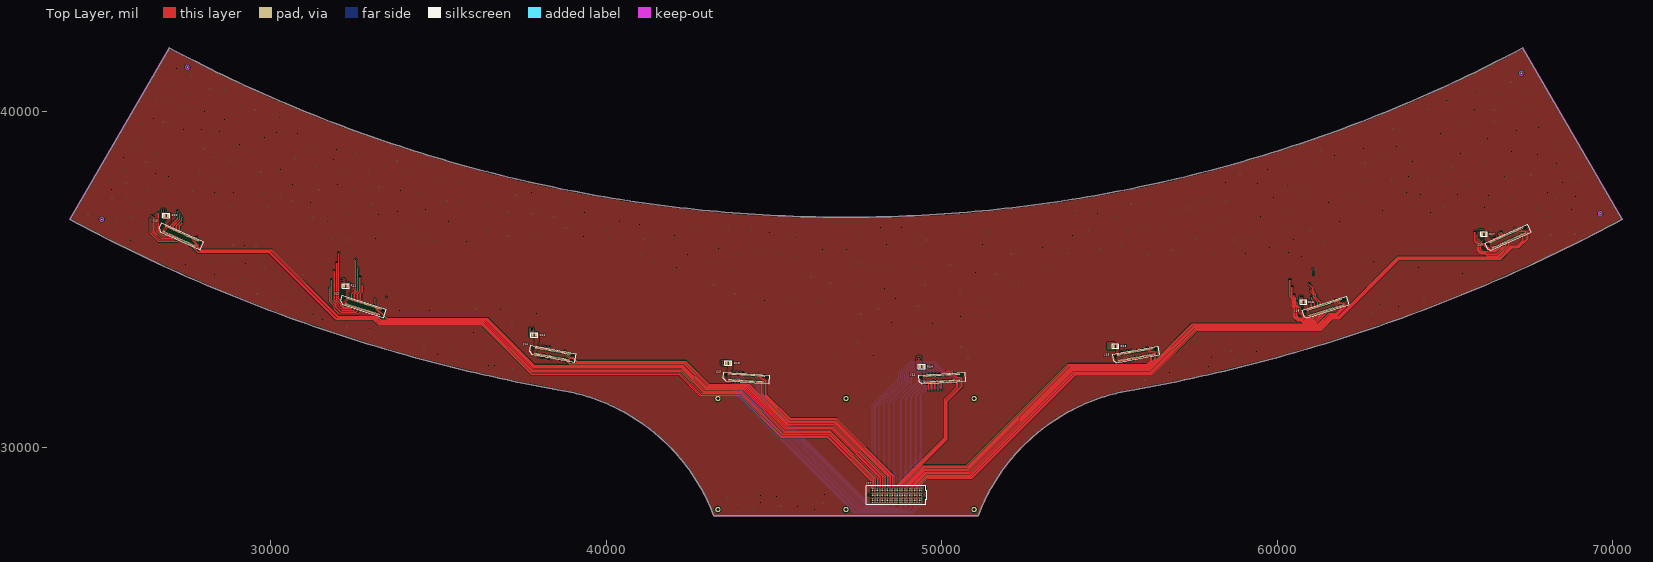
[diagram p0: Top Layer view]
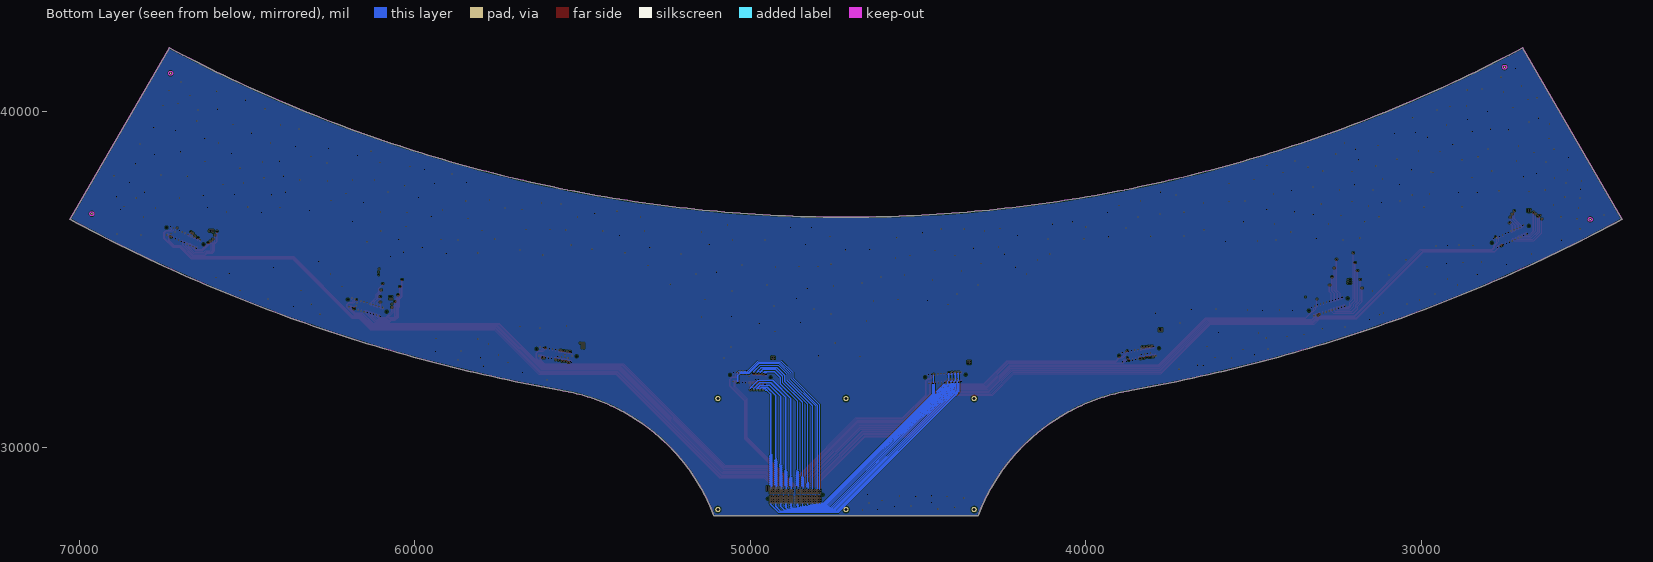
[diagram p1: Bottom Layer view, seen from below]
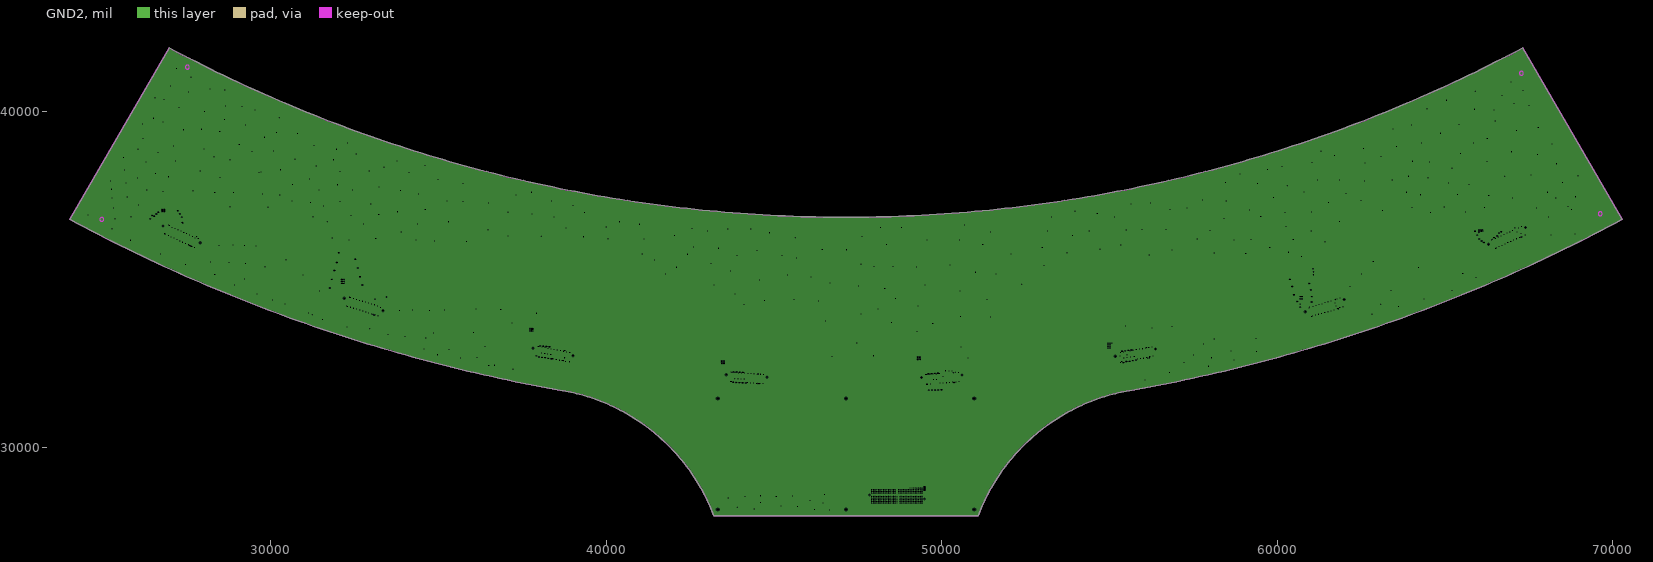
[diagram p2: GND2, clearances drawn from the general rule]
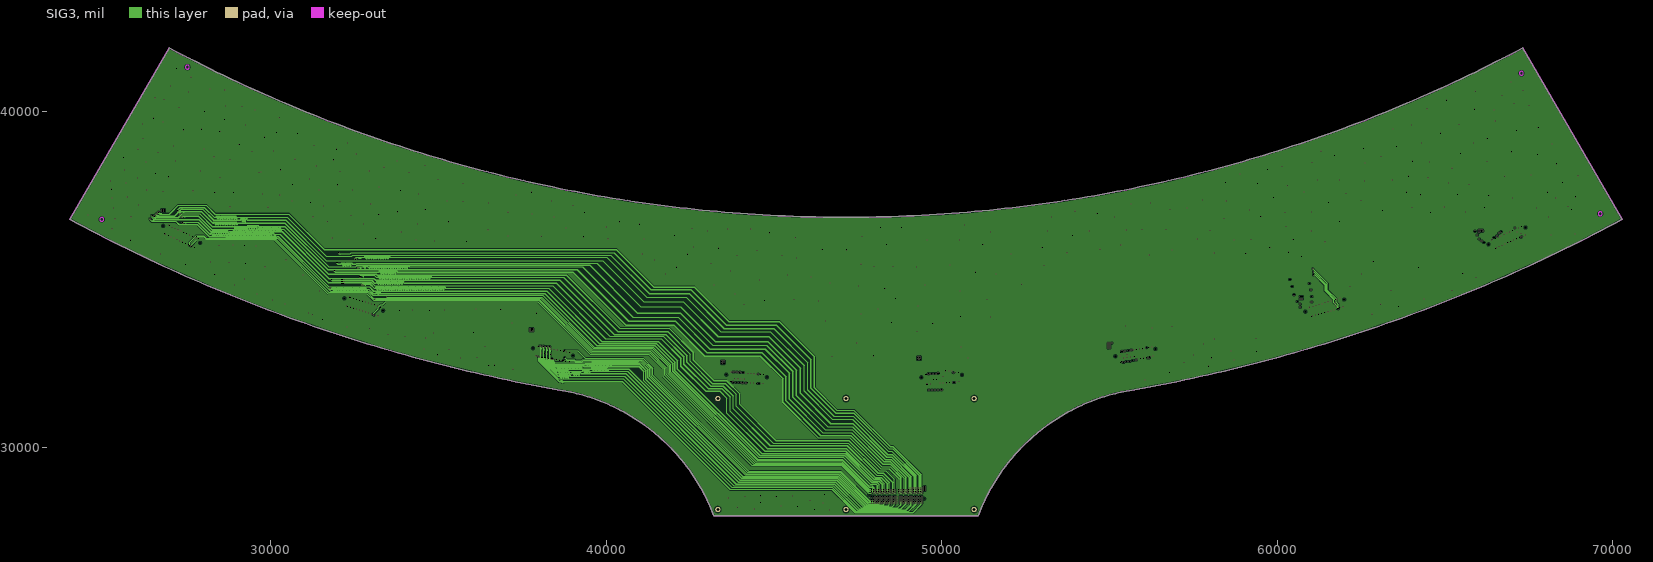
[diagram p3: SIG3]
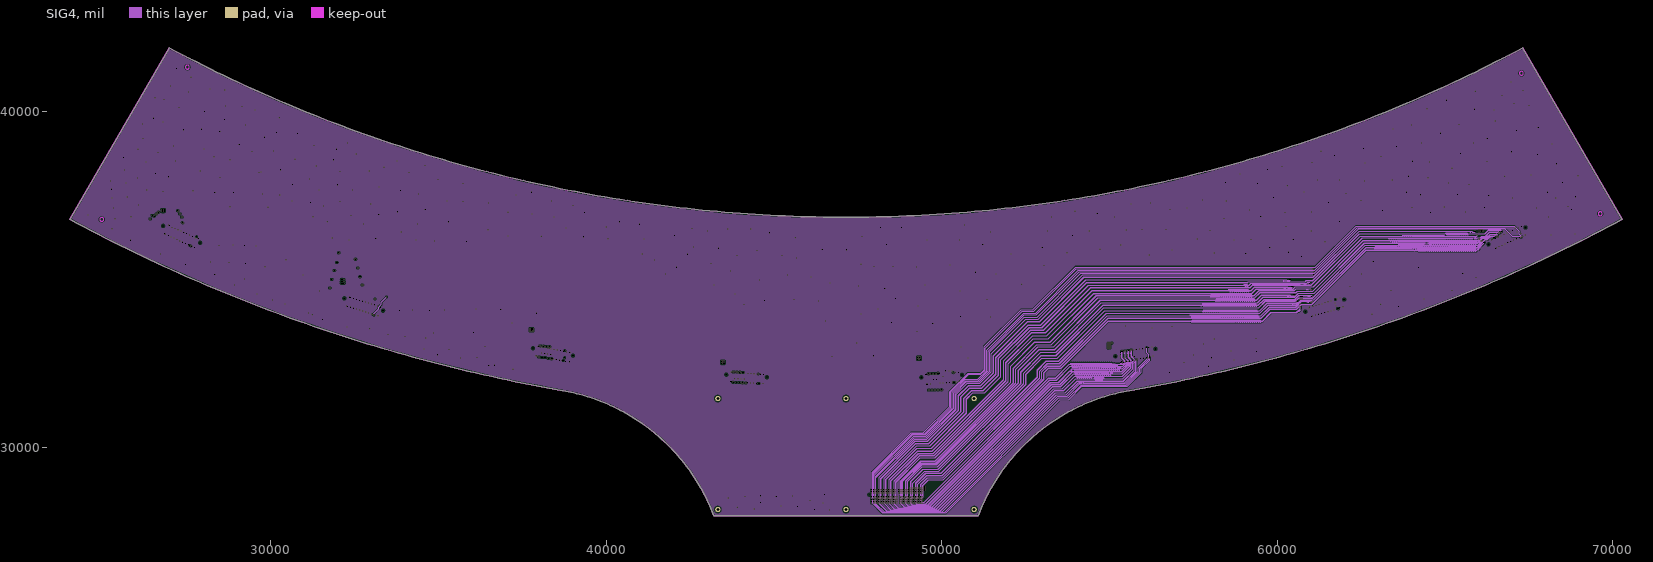
[diagram p4: SIG4]
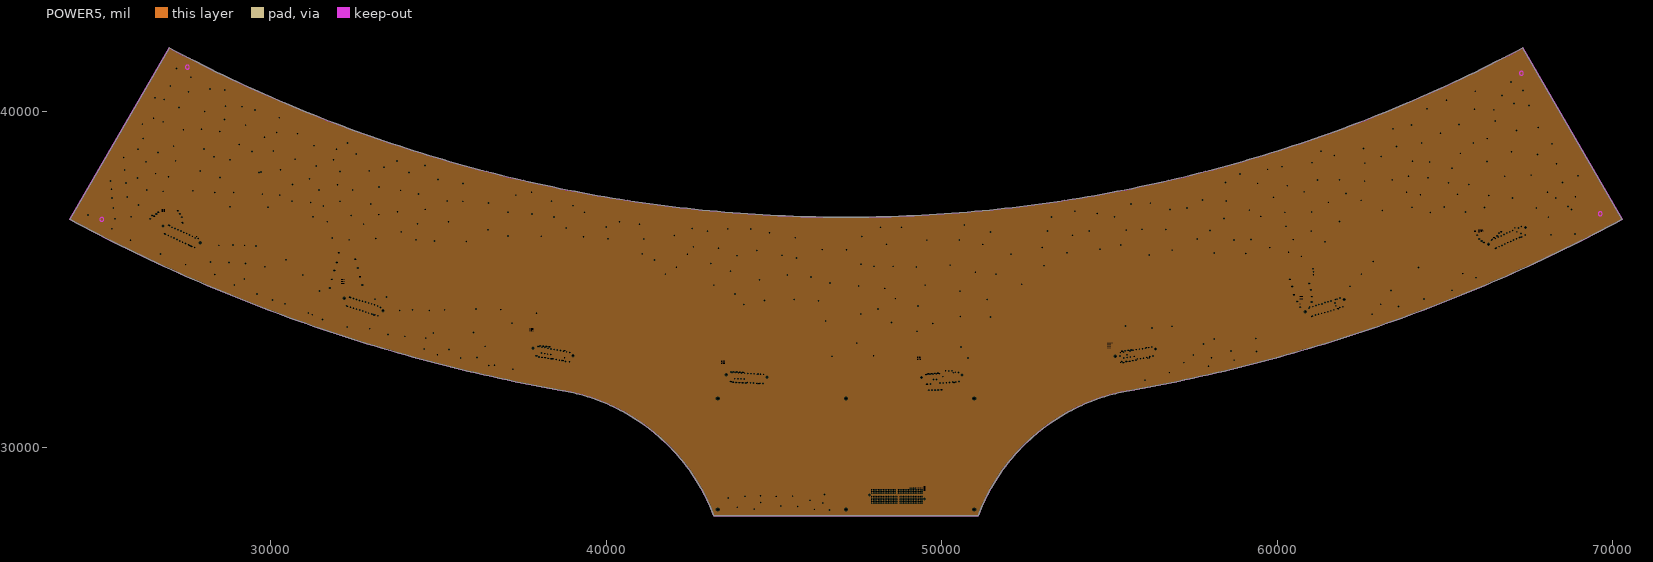
[diagram p5: POWER5, clearances drawn from the general rule]
# Altium PCB MISC86329.PcbDoc (part 1 of 11)
Units mil, origin at the board's own origin, x right, y up, seen from the top; angles counter-clockwise.
Board outline 46247.15 x 13937.21 mil, 6 copper layers (Top Layer, GND2, SIG3, SIG4, POWER5, Bottom Layer); 17 components, 210 nets, 908 pads, 1109 vias.

## Layer stack, top to bottom (the 12.6 mil dielectric is the usual default, probably not edited)
Top Layer: signal copper 1.4
Dielectric: core 12.6, FR-4, Dk 4.8
GND2: plane copper 1.4, net DGND
Dielectric: prepreg 12.6, FR-4, Dk 4.8
SIG3: signal copper 1.4
Dielectric: core 12.6, FR-4, Dk 4.8
SIG4: signal copper 1.4
Dielectric: prepreg 12.6, FR-4, Dk 4.8
POWER5: plane copper 1.4, net 5V_OUT
Dielectric: core 12.6, FR-4, Dk 4.8
Bottom Layer: signal copper 1.4

## Board outline
24025.43,36800.52 ccw(c47149,79657.81) 38712.02,31696.74 38711.64,31696.8 cw(c37688.49,25880.6) 43212,27970.07 43211.99,27970.1 51086.01,27970.1 51086,27970.07 cw(c56609.51,25880.6) 55586.37,31696.8 55585.98,31696.74 ccw(c47149,79657.81) 70272.58,36800.52 70272.27,36800.35 67306.49,41907.14 67306.76,41907.28 cw(c47149,79657.81) 26991.25,41907.28 26991.51,41907.14

## Design rules (kind name [scope] priority, off if disabled: settings)
Clearance [All] p1: gap=5
DiffPairsRouting [All] p1: maxlimit=5 minlimit=5 mostfreqgap=5 maxuncoupledlength=500
HoleToHoleClearance [All] p1: gap=0 allowstackedmicrovias=TRUE
MinimumSolderMaskSliver [All] p1: minsoldermaskwidth=0
PlaneClearance [All] p1: clearance=20
PlaneConnect [All] p1: planeconnectstyle=Direct reliefexpansion=20 reliefentries=4 reliefconductorwidth=10 reliefairgap=10
PolygonConnect PolygonConnect_1 [isvia] p1: connectstyle=Direct reliefconductorwidth=10 reliefentries=4 polygonreliefangle="90 Angle"
PolygonConnect [All] p2: connectstyle=Relief reliefconductorwidth=10 reliefentries=4 polygonreliefangle="90 Angle"
RoutingVias [All] p1: holewidth=12 width=24 viastyle="Through Hole" minholewidth=12 minwidth=24 maxholewidth=12 maxwidth=24
SilkToSilkClearance [All] p1: silktosilkclearance=0
SilkscreenOverComponentPads [All] p1: minsilkscreentomaskgap=0
SolderMaskExpansion [All] p1: expansion=4
Width [All] p1: maxlimit=20 minlimit=5 preferedwidth=5 minimp=50.000000 maximp=50.000000 favimp=50.000000
21 further rules are at their usual default settings.

## Classes and differential pairs
differential pair NewDifferentialPair1: +CLKM_CH0 -CLKP_CH0
differential pair NewDifferentialPair2: +CLKM_CH1 -CLKP_CH1
differential pair NewDifferentialPair3: +CLKM_CH2 -CLKP_CH2
differential pair NewDifferentialPair4: +CLKM_CH3 -CLKP_CH3
differential pair NewDifferentialPair5: +CLKM_CH4 -CLKP_CH4
differential pair NewDifferentialPair6: +CLKM_CH5 -CLKP_CH5
differential pair NewDifferentialPair7: +CLKM_CH6 -CLKP_CH6
differential pair NewDifferentialPair8: +CLKM_CH7 -CLKP_CH7
differential pair NewDifferentialPair9: +DATAIN0N_CH0 -DATAIN0P_CH0
differential pair NewDifferentialPair10: +DATAIN0N_CH1 -DATAIN0P_CH1
differential pair NewDifferentialPair11: +DATAIN0N_CH2 -DATAIN0P_CH2
differential pair NewDifferentialPair12: +DATAIN0N_CH3 -DATAIN0P_CH3
differential pair NewDifferentialPair13: +DATAIN0N_CH4 -DATAIN0P_CH4
differential pair NewDifferentialPair14: +DATAIN0N_CH5 -DATAIN0P_CH5
differential pair NewDifferentialPair15: +DATAIN0N_CH6 -DATAIN0P_CH6
differential pair NewDifferentialPair16: +DATAIN0N_CH7 -DATAIN0P_CH7
differential pair NewDifferentialPair17: +DATAIN1N_CH0 -DATAIN1P_CH0
differential pair NewDifferentialPair18: +DATAIN1N_CH1 -DATAIN1P_CH1
differential pair NewDifferentialPair19: +DATAIN1N_CH2 -DATAIN1P_CH2
differential pair NewDifferentialPair20: +DATAIN1N_CH3 -DATAIN1P_CH3
differential pair NewDifferentialPair21: +DATAIN1N_CH4 -DATAIN1P_CH4
differential pair NewDifferentialPair22: +DATAIN1N_CH5 -DATAIN1P_CH5
differential pair NewDifferentialPair23: +DATAIN1N_CH6 -DATAIN1P_CH6
differential pair NewDifferentialPair24: +DATAIN1N_CH7 -DATAIN1P_CH7
differential pair NewDifferentialPair25: +DATAIN2N_CH0 -DATAIN2P_CH0
differential pair NewDifferentialPair26: +DATAIN2N_CH1 -DATAIN2P_CH1
differential pair NewDifferentialPair27: +DATAIN2N_CH2 -DATAIN2P_CH2
differential pair NewDifferentialPair28: +DATAIN2N_CH3 -DATAIN2P_CH3
differential pair NewDifferentialPair29: +DATAIN2N_CH4 -DATAIN2P_CH4
differential pair NewDifferentialPair30: +DATAIN2N_CH5 -DATAIN2P_CH5
differential pair NewDifferentialPair31: +DATAIN2N_CH6 -DATAIN2P_CH6
differential pair NewDifferentialPair32: +DATAIN2N_CH7 -DATAIN2P_CH7
differential pair NewDifferentialPair33: +DATAIN3N_CH0 -DATAIN3P_CH0
differential pair NewDifferentialPair34: +DATAIN3N_CH1 -DATAIN3P_CH1
differential pair NewDifferentialPair35: +DATAIN3N_CH2 -DATAIN3P_CH2
differential pair NewDifferentialPair36: +DATAIN3N_CH3 -DATAIN3P_CH3
differential pair NewDifferentialPair37: +DATAIN3N_CH4 -DATAIN3P_CH4
differential pair NewDifferentialPair38: +DATAIN3N_CH5 -DATAIN3P_CH5
differential pair NewDifferentialPair39: +DATAIN3N_CH6 -DATAIN3P_CH6
differential pair NewDifferentialPair40: +DATAIN3N_CH7 -DATAIN3P_CH7
differential pair NewDifferentialPair41: +DATAIN4N_CH0 -DATAIN4P_CH0
differential pair NewDifferentialPair42: +DATAIN4N_CH1 -DATAIN4P_CH1
differential pair NewDifferentialPair43: +DATAIN4N_CH2 -DATAIN4P_CH2
differential pair NewDifferentialPair44: +DATAIN4N_CH3 -DATAIN4P_CH3
differential pair NewDifferentialPair45: +DATAIN4N_CH4 -DATAIN4P_CH4
differential pair NewDifferentialPair46: +DATAIN4N_CH5 -DATAIN4P_CH5
differential pair NewDifferentialPair47: +DATAIN4N_CH6 -DATAIN4P_CH6
differential pair NewDifferentialPair48: +DATAIN4N_CH7 -DATAIN4P_CH7
differential pair NewDifferentialPair49: +DATAIN5N_CH0 -DATAIN5P_CH0
differential pair NewDifferentialPair50: +DATAIN5N_CH1 -DATAIN5P_CH1
differential pair NewDifferentialPair51: +DATAIN5N_CH2 -DATAIN5P_CH2
differential pair NewDifferentialPair52: +DATAIN5N_CH3 -DATAIN5P_CH3
differential pair NewDifferentialPair53: +DATAIN5N_CH4 -DATAIN5P_CH4
differential pair NewDifferentialPair54: +DATAIN5N_CH5 -DATAIN5P_CH5
differential pair NewDifferentialPair55: +DATAIN5N_CH6 -DATAIN5P_CH6
differential pair NewDifferentialPair56: +DATAIN5N_CH7 -DATAIN5P_CH7
differential pair NewDifferentialPair57: +DATAIN6N_CH0 -DATAIN6P_CH0
differential pair NewDifferentialPair58: +DATAIN6N_CH1 -DATAIN6P_CH1
differential pair NewDifferentialPair59: +DATAIN6N_CH2 -DATAIN6P_CH2
differential pair NewDifferentialPair60: +DATAIN6N_CH3 -DATAIN6P_CH3
differential pair NewDifferentialPair61: +DATAIN6N_CH4 -DATAIN6P_CH4
differential pair NewDifferentialPair62: +DATAIN6N_CH5 -DATAIN6P_CH5
differential pair NewDifferentialPair63: +DATAIN6N_CH6 -DATAIN6P_CH6
differential pair NewDifferentialPair64: +DATAIN6N_CH7 -DATAIN6P_CH7
differential pair NewDifferentialPair65: +DATAIN7N_CH0 -DATAIN7P_CH0
differential pair NewDifferentialPair66: +DATAIN7N_CH1 -DATAIN7P_CH1
differential pair NewDifferentialPair67: +DATAIN7N_CH2 -DATAIN7P_CH2
differential pair NewDifferentialPair68: +DATAIN7N_CH3 -DATAIN7P_CH3
differential pair NewDifferentialPair69: +DATAIN7N_CH4 -DATAIN7P_CH4
differential pair NewDifferentialPair70: +DATAIN7N_CH5 -DATAIN7P_CH5
differential pair NewDifferentialPair71: +DATAIN7N_CH6 -DATAIN7P_CH6
differential pair NewDifferentialPair72: +DATAIN7N_CH7 -DATAIN7P_CH7

## Components (designator, comment, footprint, x,y, rotation, side; value= is the part's Value field where it differs from the comment)
J10 "ERF8-035-XX.X-X-DV" ERF8-035-XX.X-X-DV 27328.13,36298.88 r155.43 top
J11 "ERF8-035-XX.X-X-DV" ERF8-035-XX.X-X-DV 50003.99,32068.81 r183.43 top
J12 "ERF8-035-XX.X-X-DV" ERF8-035-XX.X-X-DV 32759.99,34206.52 r162.43 top
J13 "ERF8-035-XX.X-X-DV" ERF8-035-XX.X-X-DV 44183.07,32075.6 r176.43 top
J14 "ERF8-035-XX.X-X-DV" ERF8-035-XX.X-X-DV 38406.36,32791.72 r169.43 top locked
J15 "ERF8-035-XX.X-X-DV" ERF8-035-XX.X-X-DV 55782.35,32771.47 r190.43 top
J16 "ERF8-035-XX.X-X-DV" ERF8-035-XX.X-X-DV 61432.01,34173.09 r197.43 top
J17 "SEAF-30-XX.X-XX-10-X-A" SEAF-30-XX.X-XX-10-X-A 48662.89,28593.8 r0 top locked
J18 "ERM8-035-XX.X-X-DV" ERF8-035-XX.X-X-DV 66868.74,36252.79 r204.43 top
R10 "100R" R1210 26890,36920 r180 top
R11 "100R" R1210 32240,34820 r180 top
R12 "100R" R1210 37860,33360 r180 top
R13 "100R" R1210 43640,32520 r180 top
R14 "100R" R1210 49409,32421 r180 top
R15 "100R" R1210 55180,33020 r180 top
R16 "100R" R1210 60780,34340 r180 top
R17 "100R" R1210 66160,36360 r180 top

## Footprints (in the part's own frame and the unit in brackets; to place one, negate y for a bottom-side part, rotate by r counter-clockwise, add the part's x,y. Pads: shape width x height; smd on the part's side, far side on the other; paste and mask are expansions set on the pad)
ERF8-035-XX.X-X-DV [mm]
  rect 0.5x1.1 smd mask+0.05: 1(13.6,2.25) 2(13.6,-2.25) 3(12.8,2.25) 4(12.8,-2.25) 5(12,2.25) 6(12,-2.25) 7(11.2,2.25) 8(11.2,-2.25) 9(10.4,2.25) 10(10.4,-2.25) 11(9.6,2.25) 12(9.6,-2.25) 13(8.8,2.25) 14(8.8,-2.25) 15(8,2.25) 16(8,-2.25) 17(7.2,2.25) 18(7.2,-2.25) 19(6.4,2.25) 20(6.4,-2.25) 21(5.6,2.25) 22(5.6,-2.25) 23(4.8,2.25) 24(4.8,-2.25) 25(4,2.25) 26(4,-2.25) 27(3.2,2.25) 28(3.2,-2.25) 29(2.4,2.25) 30(2.4,-2.25) 31(1.6,2.25) 32(1.6,-2.25) 33(0.8,2.25) 34(0.8,-2.25) 35(0,2.25) 36(0,-2.25) 37(-0.8,2.25) 38(-0.8,-2.25) 39(-1.6,2.25) 40(-1.6,-2.25) 41(-2.4,2.25) 42(-2.4,-2.25) 43(-3.2,2.25) 44(-3.2,-2.25) 45(-4,2.25) 46(-4,-2.25) 47(-4.8,2.25) 48(-4.8,-2.25) 49(-5.6,2.25) 50(-5.6,-2.25) 51(-6.4,2.25) 52(-6.4,-2.25) 53(-7.2,2.25) 54(-7.2,-2.25) 55(-8,2.25) 56(-8,-2.25) 57(-8.8,2.25) 58(-8.8,-2.25) 59(-9.6,2.25) 60(-9.6,-2.25) 61(-10.4,2.25) 62(-10.4,-2.25) 63(-11.2,2.25) 64(-11.2,-2.25) 65(-12,2.25) 66(-12,-2.25) 67(-12.8,2.25) 68(-12.8,-2.25) 69(-13.6,2.25) 70(-13.6,-2.25)
  round 0 hole 1.45 unplated: MH1(15.4,-1.5) MH2(-15.4,-1.5)
  silkscreen extent -17.51,-3.3 17.51,3.3
R1210 [mm] "Chip Capacitor; Body 3.2 x 2.5 mm (LxW typ)"
  rect 1.6x2.7 smd: 1(-1.4,0) 2(1.4,0)
  silkscreen extent -2.6,-1.7 2.6,1.7
SEAF-30-XX.X-XX-10-X-A [mil]
  round 25 smd paste+5 mask+2: A1(725,-225) A2(675,-225) A3(625,-225) A4(575,-225) A5(525,-225) A6(475,-225) A7(425,-225) A8(375,-225) A9(325,-225) A10(275,-225) A11(225,-225) A12(175,-225) A13(125,-225) A14(75,-225) A15(25,-225) A16(-25,-225) A17(-75,-225) A18(-125,-225) A19(-175,-225) A20(-225,-225) A21(-275,-225) A22(-325,-225) A23(-375,-225) A24(-425,-225) A25(-475,-225) A26(-525,-225) A27(-575,-225) A28(-625,-225) A29(-675,-225) A30(-725,-225) B1(725,-175) B2(675,-175) B3(625,-175) B4(575,-175) B5(525,-175) B6(475,-175) B7(425,-175) B8(375,-175) B9(325,-175) B10(275,-175) B11(225,-175) B12(175,-175) B13(125,-175) B14(75,-175) B15(25,-175) B16(-25,-175) B17(-75,-175) B18(-125,-175) B19(-175,-175) B20(-225,-175) B21(-275,-175) B22(-325,-175) B23(-375,-175) B24(-425,-175) B25(-475,-175) B26(-525,-175) B27(-575,-175) B28(-625,-175) B29(-675,-175) B30(-725,-175) C1(725,-125) C2(675,-125) C3(625,-125) C4(575,-125) C5(525,-125) C6(475,-125) C7(425,-125) C8(375,-125) C9(325,-125) C10(275,-125) C11(225,-125) C12(175,-125) C13(125,-125) C14(75,-125) C15(25,-125) C16(-25,-125) C17(-75,-125) C18(-125,-125) C19(-175,-125) C20(-225,-125) C21(-275,-125) C22(-325,-125) C23(-375,-125) C24(-425,-125) C25(-475,-125) C26(-525,-125) C27(-575,-125) C28(-625,-125) C29(-675,-125) C30(-725,-125) D1(725,-75) D2(675,-75) D3(625,-75) D4(575,-75) D5(525,-75) D6(475,-75) D7(425,-75) D8(375,-75) D9(325,-75) D10(275,-75) D11(225,-75) D12(175,-75) D13(125,-75) D14(75,-75) D15(25,-75) D16(-25,-75) D17(-75,-75) D18(-125,-75) D19(-175,-75) D20(-225,-75) D21(-275,-75) D22(-325,-75) D23(-375,-75) D24(-425,-75) D25(-475,-75) D26(-525,-75) D27(-575,-75) D28(-625,-75) D29(-675,-75) D30(-725,-75) E1(725,-25) E2(675,-25) E3(625,-25) E4(575,-25) E5(525,-25) E6(475,-25) E7(425,-25) E8(375,-25) E9(325,-25) E10(275,-25) E11(225,-25) E12(175,-25) E13(125,-25) E14(75,-25) E15(25,-25) E16(-25,-25) E17(-75,-25) E18(-125,-25) E19(-175,-25) E20(-225,-25) E21(-275,-25) E22(-325,-25) E23(-375,-25) E24(-425,-25) E25(-475,-25) E26(-525,-25) E27(-575,-25) E28(-625,-25) E29(-675,-25) E30(-725,-25) F1(725,25) F2(675,25) F3(625,25) F4(575,25) F5(525,25) F6(475,25) F7(425,25) F8(375,25) F9(325,25) F10(275,25) F11(225,25) F12(175,25) F13(125,25) F14(75,25) F15(25,25) F16(-25,25) F17(-75,25) F18(-125,25) F19(-175,25) F20(-225,25) F21(-275,25) F22(-325,25) F23(-375,25) F24(-425,25) F25(-475,25) F26(-525,25) F27(-575,25) F28(-625,25) F29(-675,25) F30(-725,25) G1(725,75) G2(675,75) G3(625,75) G4(575,75) G5(525,75) G6(475,75) G7(425,75) G8(375,75) G9(325,75) G10(275,75) G11(225,75) G12(175,75) G13(125,75) G14(75,75) G15(25,75) G16(-25,75) G17(-75,75) G18(-125,75) G19(-175,75) G20(-225,75) G21(-275,75) G22(-325,75) G23(-375,75) G24(-425,75) G25(-475,75) G26(-525,75) G27(-575,75) G28(-625,75) G29(-675,75) G30(-725,75) H1(725,125) H2(675,125) H3(625,125) H4(575,125) H5(525,125) H6(475,125) H7(425,125) H8(375,125) H9(325,125) H10(275,125) H11(225,125) H12(175,125) H13(125,125) H14(75,125) H15(25,125) H16(-25,125) H17(-75,125) H18(-125,125) H19(-175,125) H20(-225,125) H21(-275,125) H22(-325,125) H23(-375,125) H24(-425,125) H25(-475,125) H26(-525,125) H27(-575,125) H28(-625,125) H29(-675,125) H30(-725,125) J1(725,175) J2(675,175) J3(625,175) J4(575,175) J5(525,175) J6(475,175) J7(425,175) J8(375,175) J9(325,175) J10(275,175) J11(225,175) J12(175,175) J13(125,175) J14(75,175) J15(25,175) J16(-25,175) J17(-75,175) J18(-125,175) J19(-175,175) J20(-225,175) J21(-275,175) J22(-325,175) J23(-375,175) J24(-425,175) J25(-475,175) J26(-525,175) J27(-575,175) J28(-625,175) J29(-675,175) J30(-725,175) K1(725,225) K2(675,225) K3(625,225) K4(575,225) K5(525,225) K6(475,225) K7(425,225) K8(375,225) K9(325,225) K10(275,225) K11(225,225) K12(175,225) K13(125,225) K14(75,225) K15(25,225) K16(-25,225) K17(-75,225) K18(-125,225) K19(-175,225) K20(-225,225) K21(-275,225) K22(-325,225) K23(-375,225) K24(-425,225) K25(-475,225) K26(-525,225) K27(-575,225) K28(-625,225) K29(-675,225) K30(-725,225)
  round 0 hole 50 unplated: MH1(820.5,-120) MH2(-820.5,0)
  silkscreen extent -905,-280 895,280

## Part data
J10 J11 J12 J13 J14 J15 J16: "0.8mm Edge Rate Socket Assembly, Double Vertical Row, 30 Positions Per Row."
J17: "Socket Array Assembly, Surface Mount, 0.050\" Pitch, 300 Pins"
J18: "0.8mm Edge Rate Terminal Assembly, Double Vertical Row, 40 Position, 0.8mm Pitch"
R10 R11 R12 R13 R14 R15 R16 R17: library part Res_4K7_0.05_1608[0603]_FENGHUA, "Resistor"

## Free pads (board coordinates)
  round 39.37 smd mask+39.37: 0(24972,36798) 0(27525,41336) 0(67272,41153) 0(69620,36968)
  round 39.37 smd far side mask+39.37: 0(24972,36798) 0(27525,41336) 0(67272,41153) 0(69620,36968)
  round 157.48 hole 86.61: 0(43330,28152.91) 0(43330,31460) 0(47148.9,28152.91) 0(47148.9,31460) 0(50967.8,28152.91) 0(50967.8,31460)

## Via types
v1: diameter 24, hole 12, Top Layer to Bottom Layer, 684 vias
v2: diameter 18, hole 9, Top Layer to Bottom Layer, 425 vias

## Nets (pads, with @x,y where several pads share a name; then routed paths per layer and width w, separated by ;. In a path a pad name is that pad's centre, name@x,y a point inside that pad or via, vN(x,y) a via of type N, cw(c..) or ccw(c..) an arc to the next point about the centre after c; other vN are vias at no path point)
5V_OUT: J17.J1 J17.J2 J17.J3 J17.J4 R10.2 R11.2 R12.2 R13.2 R14.2 R15.2 R16.2 R17.2 | length 134.7
  Top Layer w20: J17.J4@49237.89,28768.8 v2(49261.69,28792.61) ; J17.J3@49287.89,28768.8 v2(49311.69,28792.61) ; J17.J2@49337.89,28768.8 v2(49361.69,28792.61) ; J17.J1@49387.89,28768.8 v2(49411.69,28792.61)
  other v1: 49475,28725 49502,28726 49475,28750 49501,28752 49475,28776 49502,28777 49475,28805 49503,28807 49474,28833 49502,28834 43481,32500 43443,32502 43520,32502 43520,32541 43479,32542 43440,32545 43522,32579 43440,32580 43479,32580 49283,32623 49319,32623 49363,32624 49281,32663 49320,32664 49362,32664 49280,32702 49319,32702 49359,32703 54958,32962 55013,32965 54959,33015 55012,33017 54955,33063 55012,33064 54958,33107 55013,33107 55071,33110 37777,33473 37817,33474 37736,33476 37774,33511 37737,33512 37815,33513 37736,33548 37774,33548 37815,33548 60681,34274 60680,34432 60712,34432 60745,34432 60682,34497 60715,34497 60745,34497 32153,34893 32197,34893 32112,34894 32112,34951 32197,34951 32151,34952 32190,35009 32113,35011 32151,35011 66005,36411 66003,36446 66046,36447 66086,36447 66124,36448 66040,36480 66076,36480 66004,36481 66117,36481 26767,37030 26803,37030 26842,37031 26801,37064 26842,37065 26766,37066 26800,37094 26764,37095 26840,37095
  other v2: 49311.69,28792.61
5V_POWERIN0: J10.1 J10.2 J10.3 J10.4 R10.1
5V_POWERIN1: J12.1 J12.2 J12.3 J12.4 R11.1
5V_POWERIN2: J14.1 J14.2 J14.3 J14.4 R12.1
5V_POWERIN3: J13.1 J13.2 J13.3 J13.4 R13.1
5V_POWERIN4: J11.1 J11.2 J11.3 J11.4 R14.1
5V_POWERIN5: J15.1 J15.2 J15.3 J15.4 R15.1
5V_POWERIN6: J16.1 J16.2 J16.3 J16.4 R16.1
5V_POWERIN7: J18.1 J18.2 J18.3 J18.4 R17.1
CLKM_CH0: J10.11 J17.G2 | length 28227.1
  Top Layer w5: v2(26648.5,37013) 26655,37006.5 26655,36454.86 26787.86,36322 26908.14,36322 26928.92,36342.78 26928.92,36356.83 J10.11@26947.56,36375.47 ; J17.G2@49337.89,28668.8 v2(49361.69,28692.61)
  SIG3 w5: v2(26648.5,37013) 26655,37006.5 26655,36987 26694,36948 26993.14,36948 27054,37008.86 27054,37009 ; 27053,37008 27259,37214 28080.86,37214 28346.86,36948 30545.86,36948 31601.86,35892 40305,35892 41416,34781 42621.86,34781 43650.86,33752 45157,33752 46202,32707 46202,31778.86 46875.86,31105 47382.86,31105 48461.86,30026 48543,30026 49381.69,29187.31 49381.69,28712.61 v2(49361.69,28692.61)
CLKM_CH1: J12.11 J17.F2 | length 23095.3
  Top Layer w5: v2(32022.5,35804) 32029,35797.5 32029,34427.86 32134,34322.86 32134,34231.86 32199.86,34166 32329.14,34166 32352.9,34189.76 32352.9,34216.13 J12.11@32372.93,34236.16 ; J17.F2@49337.89,28618.8 v2(49361.69,28642.61)
  SIG3 w5: v2(32022.5,35804) 32029,35797.5 32029,35780.86 32040.86,35769 32061,35769 32067,35763 32080,35763 32086,35769 32382.14,35769 32412.14,35799 40234.86,35799 40238.86,35795 40239,35795 ; 40238.93,35794.93 41330.86,34703 42517.86,34703 43574.86,33646 45069,33646 46099,32616 46099,31766.86 46840.86,31025 47372.86,31025 48439.86,29958 48535,29958 49333,29160 49333,28664.86 49343.86,28654 49350.3,28654 v2(49361.69,28642.61)
CLKM_CH2: J14.11 J17.B2 | length 13806.2
  Top Layer w5: v2(38013.5,32699) 38007,32705.5 38007,32745 38018.58,32756.58 J14.11@38018.58,32773.97 ; J17.B2@49337.89,28418.8 v2(49361.69,28395)
  SIG3 w5: v2@38012,32696 38007,32691 38007,32673 38011.5,32668.5 38025.75,32668.5 38032,32662.25 38032,32649.75 38025.75,32643.5 38011.5,32643.5 38007,32639 38007,32572.14 38602.14,31977 38643.68,31977 38649.5,31982.82 38649.5,31997.38 38661.18,32009.06 38682.82,32009.06 38694.5,31997.38 38694.5,31950.76 38700.32,31944.94 38713.68,31944.94 38719.5,31950.76 38719.5,31965.32 38731.18,31977 40479,31977 43693,28763 46733,28763 47421,28075 49148.69,28075 49381.69,28308 49381.69,28375 v2(49361.69,28395)
CLKM_CH3: J13.11 J17.A2 | length 7749.2
  Top Layer w5: 43789.62,31951.5 43789.62,31974.28 43800.33,31985 J13.11@43800.33,32010.72 ; J17.A2@49337.89,28368.8 v2(49361.69,28345)
  Bottom Layer w5: v2(43796.12,31945) 43790,31938.88 43790,31903.25 43793.75,31899.5 43799.11,31899.5 43802.86,31895.75 43802.86,31878.25 43799.11,31874.5 43793.75,31874.5 43790,31870.75 43790,31853.25 43793.75,31849.5 43799.11,31849.5 43802.86,31845.75 43802.86,31828.25 43799.11,31824.5 43793.75,31824.5 43790,31820.75 43790,31674 43807.57,31656.43 43814.04,31656.43 43817.57,31659.96 43832.32,31659.96 43842.32,31649.96 43842.32,31635.22 43824.64,31617.54 43824.64,31611.07 43828.78,31606.93 43835.25,31606.93 43852.93,31624.61 43867.68,31624.61 43877.68,31614.61 43877.68,31599.86 43860,31582.18 43860,31575.72 43864.14,31571.58 43870.6,31571.58 43874.14,31575.11 43888.89,31575.11 47389,28075 49155.86,28075 49381.69,28300.83 49381.69,28325 v2(49361.69,28345)
CLKM_CH4: J11.11 J17.H2 | length 5095.5
  Top Layer w5: J17.H2@49337.89,28718.8 v2(49361.69,28742.61) ; 49621.3,31719.5 49621.3,31922.28 49632.02,31933 J11.11@49632.02,31957.77
  Bottom Layer w5: v2(49361.69,28742.61) 49381.69,28762.61 49381.69,28847.93 49378.62,28851 49360.62,28851 49351.69,28859.93 49351.69,28882.07 49360.62,28891 49408.62,28891 49411.69,28894.07 49411.69,28907.93 49408.62,28911 49360.62,28911 49351.69,28919.93 49351.69,28942.07 49360.62,28951 49408.62,28951 49411.69,28954.07 49411.69,28967.93 49408.62,28971 49360.62,28971 49351.69,28979.93 49351.69,29002.07 49360.62,29011 49408.62,29011 49411.69,29014.07 49411.69,29027.93 49408.62,29031 49360.62,29031 49351.69,29039.93 49351.69,29062.07 49360.62,29071 49408.62,29071 49411.69,29074.07 49411.69,29087.93 49408.62,29091 49360.62,29091 49351.69,29099.93 49351.69,29122.07 49360.62,29131 49408.62,29131 49411.69,29134.07 49411.69,29147.93 49408.62,29151 49360.62,29151 49351.69,29159.93 49351.69,29182.07 49360.62,29191 49408.62,29191 49411.69,29194.07 49411.69,29207.93 49408.62,29211 49360.62,29211 49351.69,29219.93 49351.69,29242.07 49360.62,29251 49408.62,29251 49411.69,29254.07 49411.69,29267.93 49408.62,29271 49360.62,29271 49351.69,29279.93 49351.69,29302.07 49360.62,29311 49408.62,29311 49411.69,29314.07 49411.69,29327.93 49408.62,29331 49360.62,29331 49351.69,29339.93 49351.69,29362.07 49360.62,29371 49408.62,29371 49411.69,29374.07 49411.69,29387.93 49408.62,29391 49360.62,29391 49351.69,29399.93 49351.69,29422.07 49360.62,29431 49408.62,29431 49411.69,29434.07 49411.69,29447.93 49408.62,29451 49360.62,29451 49351.69,29459.93 49351.69,29482.07 49360.62,29491 49408.62,29491 49411.69,29494.07 49411.69,29507.93 49408.62,29511 49360.62,29511 49351.69,29519.93 49351.69,29542.07 49360.62,29551 49408.62,29551 49411.69,29554.07 49411.69,29567.93 49408.62,29571 49360.62,29571 49351.69,29579.93 49351.69,29602.07 49360.62,29611 49408.62,29611 49411.69,29614.07 49411.69,29627.93 49408.62,29631 49360.62,29631 49351.69,29639.93 49351.69,29662.07 49360.62,29671 49408.62,29671 49411.69,29674.07 49411.69,29687.93 49408.62,29691 49360.62,29691 49351.69,29699.93 49351.69,29722.07 49360.62,29731 49408.62,29731 49411.69,29734.07 49411.69,29747.93 49408.62,29751 49360.62,29751 49351.69,29759.93 49351.69,29782.07 49360.62,29791 49378.62,29791 49381.69,29794.07 49381.69,31587.83 49463.43,31669.57 49499.68,31705.82 49540.86,31747 49608,31747 49621,31734 49621,31721 49624,31718 v2@49624,31717 ; v2@49624,31716 v2@49624,31717 ; v2@49624.5,31716.5 v2@49624,31717
  other v2: 49627.8,31713
CLKM_CH5: J15.11 J17.C2 | length 10127.2
  Top Layer w5: J17.C2@49337.89,28468.8 v2(49361.69,28445) ; 55419,32537.5 55419,32582.32 55426.68,32590 J15.11@55426.68,32615.93
  SIG4 w5: v2(49361.69,28445) 49381,28425.69 49381,28388.22 49404.22,28365 49483.14,28365 53187.14,32069 53397.14,32069 53806.14,32478 53840.57,32478 53851,32488.43 53851,32503.43 53855.57,32508 53866.43,32508 53871,32503.43 53871,32458.43 53881.43,32448 53900.57,32448 53911,32458.43 53911,32503.43 53915.57,32508 53926.43,32508 53931,32503.43 53931,32458.43 53941.43,32448 53960.57,32448 53971,32458.43 53971,32503.43 53975.57,32508 53986.43,32508 53991,32503.43 53991,32458.43 54001.43,32448 54020.57,32448 54031,32458.43 54031,32503.43 54035.57,32508 54046.43,32508 54051,32503.43 54051,32458.43 54061.43,32448 54080.57,32448 54091,32458.43 54091,32503.43 54095.57,32508 54106.43,32508 54111,32503.43 54111,32458.43 54121.43,32448 54140.57,32448 54151,32458.43 54151,32503.43 54155.57,32508 54166.43,32508 54171,32503.43 54171,32458.43 54181.43,32448 54200.57,32448 54211,32458.43 54211,32503.43 54215.57,32508 54226.43,32508 54231,32503.43 54231,32458.43 54241.43,32448 54260.57,32448 54271,32458.43 54271,32503.43 54275.57,32508 54286.43,32508 54291,32503.43 54291,32458.43 54301.43,32448 54320.57,32448 54331,32458.43 54331,32503.43 54335.57,32508 54346.43,32508 54351,32503.43 54351,32458.43 54361.43,32448 54380.57,32448 54391,32458.43 54391,32503.43 54395.57,32508 54406.43,32508 54411,32503.43 54411,32458.43 54421.43,32448 54440.57,32448 54451,32458.43 54451,32503.43 54455.57,32508 54466.43,32508 54471,32503.43 54471,32458.43 54481.43,32448 54500.57,32448 54511,32458.43 54511,32503.43 54515.57,32508 54526.43,32508 54531,32503.43 54531,32458.43 54541.43,32448 54560.57,32448 54571,32458.43 54571,32503.43 54575.57,32508 54586.43,32508 54591,32503.43 54591,32458.43 54601.43,32448 54620.57,32448 54631,32458.43 54631,32503.43 54635.57,32508 54646.43,32508 54651,32503.43 54651,32458.43 54661.43,32448 54680.57,32448 54691,32458.43 54691,32503.43 54695.57,32508 54706.43,32508 54711,32503.43 54711,32458.43 54721.43,32448 54740.57,32448 54751,32458.43 54751,32503.43 54755.57,32508 54766.43,32508 54771,32503.43 54771,32458.43 54781.43,32448 54800.57,32448 54811,32458.43 54811,32503.43 54815.57,32508 54826.43,32508 54831,32503.43 54831,32458.43 54841.43,32448 54860.57,32448 54871,32458.43 54871,32503.43 54875.57,32508 54886.43,32508 54891,32503.43 54891,32458.43 54901.43,32448 54920.57,32448 54931,32458.43 54931,32503.43 54935.57,32508 54946.43,32508 54951,32503.43 54951,32458.43 54961.43,32448 54980.57,32448 54991,32458.43 54991,32503.43 54995.57,32508 55006.43,32508 55011,32503.43 55011,32458.43 55021.43,32448 55040.57,32448 55051,32458.43 55051,32503.43 55055.57,32508 55066.43,32508 55071,32503.43 55071,32458.43 55081.43,32448 55100.57,32448 55111,32458.43 55111,32472.86 55131.14,32493 55147,32493 55162,32478 55397,32478 55419,32500 55419,32524 v2@55425,32530
  other v2: 55425.5,32531
CLKM_CH6: J16.11 J17.D2 | length 18298.8
  Top Layer w5: J17.D2@49337.89,28518.8 v2(49361.69,28495) ; v2(60672.5,34183) 60679,34176.5 60679,34045.86 60868.86,33856 61041.14,33856 61097,33911.86 61097,33948.06 61097.94,33949 J16.11@61097.94,33975.36
  SIG4 w5: v2(49361.69,28495) 49395,28495 49395.19,28495.19 49395.19,28501.83 49404.86,28511.5 49411.5,28511.5 49436,28536 49436,28879 49604,29047 50050,29047 53048,32045 53048,32236 53186,32374 53559.86,32374 54964.86,33779 57434.57,33779 57445,33768.57 57445,33753.57 57449.57,33749 57460.43,33749 57465,33753.57 57465,33798.57 57475.43,33809 57494.57,33809 57505,33798.57 57505,33753.57 57509.57,33749 57520.43,33749 57525,33753.57 57525,33798.57 57535.43,33809 57554.57,33809 57565,33798.57 57565,33753.57 57569.57,33749 57580.43,33749 57585,33753.57 57585,33798.57 57595.43,33809 57614.57,33809 57625,33798.57 57625,33753.57 57629.57,33749 57640.43,33749 57645,33753.57 57645,33798.57 57655.43,33809 57674.57,33809 57685,33798.57 57685,33753.57 57689.57,33749 57700.43,33749 57705,33753.57 57705,33798.57 57715.43,33809 57734.57,33809 57745,33798.57 57745,33753.57 57749.57,33749 57760.43,33749 57765,33753.57 57765,33798.57 57775.43,33809 57794.57,33809 57805,33798.57 57805,33753.57 57809.57,33749 57820.43,33749 57825,33753.57 57825,33798.57 57835.43,33809 57854.57,33809 57865,33798.57 57865,33753.57 57869.57,33749 57880.43,33749 57885,33753.57 57885,33798.57 57895.43,33809 57914.57,33809 57925,33798.57 57925,33753.57 57929.57,33749 57940.43,33749 57945,33753.57 57945,33798.57 57955.43,33809 57974.57,33809 57985,33798.57 57985,33753.57 57989.57,33749 58000.43,33749 58005,33753.57 58005,33798.57 58015.43,33809 58034.57,33809 58045,33798.57 58045,33753.57 58049.57,33749 58060.43,33749 58065,33753.57 58065,33798.57 58075.43,33809 58094.57,33809 58105,33798.57 58105,33753.57 58109.57,33749 58120.43,33749 58125,33753.57 58125,33798.57 58135.43,33809 58154.57,33809 58165,33798.57 58165,33753.57 58169.57,33749 58180.43,33749 58185,33753.57 58185,33798.57 58195.43,33809 58214.57,33809 58225,33798.57 58225,33753.57 58229.57,33749 58240.43,33749 58245,33753.57 58245,33798.57 58255.43,33809 58274.57,33809 58285,33798.57 58285,33753.57 58289.57,33749 58300.43,33749 58305,33753.57 58305,33798.57 58315.43,33809 58334.57,33809 58345,33798.57 58345,33753.57 58349.57,33749 58360.43,33749 58365,33753.57 58365,33798.57 58375.43,33809 58394.57,33809 58405,33798.57 58405,33753.57 58409.57,33749 58420.43,33749 58425,33753.57 58425,33798.57 58435.43,33809 58454.57,33809 58465,33798.57 58465,33753.57 58469.57,33749 58480.43,33749 58485,33753.57 58485,33798.57 58495.43,33809 58514.57,33809 58525,33798.57 58525,33753.57 58529.57,33749 58540.43,33749 58545,33753.57 58545,33798.57 58555.43,33809 58574.57,33809 58585,33798.57 58585,33753.57 58589.57,33749 58600.43,33749 58605,33753.57 58605,33798.57 58615.43,33809 58634.57,33809 58645,33798.57 58645,33753.57 58649.57,33749 58660.43,33749 58665,33753.57 58665,33798.57 58675.43,33809 58694.57,33809 58705,33798.57 58705,33753.57 58709.57,33749 58720.43,33749 58725,33753.57 58725,33798.57 58735.43,33809 58754.57,33809 58765,33798.57 58765,33753.57 58769.57,33749 58780.43,33749 58785,33753.57 58785,33798.57 58795.43,33809 58814.57,33809 58825,33798.57 58825,33753.57 58829.57,33749 58840.43,33749 58845,33753.57 58845,33798.57 58855.43,33809 58874.57,33809 58885,33798.57 58885,33753.57 58889.57,33749 58900.43,33749 58905,33753.57 58905,33798.57 58915.43,33809 58934.57,33809 58945,33798.57 58945,33753.57 58949.57,33749 58960.43,33749 58965,33753.57 58965,33798.57 58975.43,33809 58994.57,33809 59005,33798.57 59005,33753.57 59009.57,33749 59020.43,33749 59025,33753.57 59025,33798.57 59035.43,33809 59054.57,33809 59065,33798.57 59065,33753.57 59069.57,33749 59080.43,33749 59085,33753.57 59085,33798.57 59095.43,33809 59114.57,33809 59125,33798.57 59125,33753.57 59129.57,33749 59140.43,33749 59145,33753.57 59145,33798.57 59155.43,33809 59174.57,33809 59185,33798.57 59185,33753.57 59189.57,33749 59200.43,33749 59205,33753.57 59205,33798.57 59215.43,33809 59234.57,33809 59245,33798.57 59245,33753.57 59249.57,33749 59260.43,33749 59265,33753.57 59265,33798.57 59275.43,33809 59294.57,33809 59305,33798.57 59305,33753.57 59309.57,33749 59320.43,33749 59325,33753.57 59325,33798.57 59335.43,33809 59354.57,33809 59365,33798.57 59365,33753.57 59369.57,33749 59380.43,33749 59385,33753.57 59385,33798.57 59395.43,33809 59414.57,33809 59425,33798.57 59425,33753.57 59429.57,33749 59440.43,33749 59445,33753.57 59445,33798.57 59455.43,33809 59474.57,33809 59485,33798.57 59485,33753.57 59489.57,33749 59500.43,33749 59505,33753.57 59505,33768.57 59515.43,33779 59560,33779 59810,34029 60572,34029 60679,34136 60679,34175 v2@60674,34180
CLKM_CH7: J17.E2 J18.11 | length 23895.5
  Top Layer w5: J17.E2@49337.89,28568.8 v2(49361.69,28545) ; v2@66149,36106.5 66149,36090.86 66355.86,35884 66514.14,35884 66568,35937.86 66568,35981.52 66561.26,35988.26 J18.11@66561.26,36015.82
  SIG4 w5: v2(49361.69,28545) 49381.69,28565 49381.69,28913.69 49576,29108 50032,29108 52978,32054 52978,32257 53155,32434 53530,32434 54958,33862 59515,33862 59791,34138 60583,34138 60715,34270 61030,34270 62650,35890 64058,35890 64076,35872 64103,35872 64121,35890 64171.43,35890 64176,35894.57 64176,35909.57 64186.43,35920 64205.57,35920 64216,35909.57 64216,35864.57 64220.57,35860 64231.43,35860 64236,35864.57 64236,35909.57 64246.43,35920 64265.57,35920 64276,35909.57 64276,35864.57 64280.57,35860 64291.43,35860 64296,35864.57 64296,35909.57 64306.43,35920 64325.57,35920 64336,35909.57 64336,35864.57 64340.57,35860 64351.43,35860 64356,35864.57 64356,35909.57 64366.43,35920 64385.57,35920 64396,35909.57 64396,35864.57 64400.57,35860 64411.43,35860 64416,35864.57 64416,35909.57 64426.43,35920 64445.57,35920 64456,35909.57 64456,35864.57 64460.57,35860 64471.43,35860 64476,35864.57 64476,35909.57 64486.43,35920 64505.57,35920 64516,35909.57 64516,35864.57 64520.57,35860 64531.43,35860 64536,35864.57 64536,35909.57 64546.43,35920 64565.57,35920 64576,35909.57 64576,35864.57 64580.57,35860 64591.43,35860 64596,35864.57 64596,35909.57 64606.43,35920 64625.57,35920 64636,35909.57 64636,35864.57 64640.57,35860 64651.43,35860 64656,35864.57 64656,35909.57 64666.43,35920 64685.57,35920 64696,35909.57 64696,35864.57 64700.57,35860 64711.43,35860 64716,35864.57 64716,35909.57 64726.43,35920 64745.57,35920 64756,35909.57 64756,35864.57 64760.57,35860 64771.43,35860 64776,35864.57 64776,35909.57 64786.43,35920 64805.57,35920 64816,35909.57 64816,35864.57 64820.57,35860 64831.43,35860 64836,35864.57 64836,35909.57 64846.43,35920 64865.57,35920 64876,35909.57 64876,35864.57 64880.57,35860 64891.43,35860 64896,35864.57 64896,35909.57 64906.43,35920 64925.57,35920 64936,35909.57 64936,35864.57 64940.57,35860 64951.43,35860 64956,35864.57 64956,35909.57 64966.43,35920 64985.57,35920 64996,35909.57 64996,35864.57 65000.57,35860 65011.43,35860 65016,35864.57 65016,35909.57 65026.43,35920 65045.57,35920 65056,35909.57 65056,35864.57 65060.57,35860 65071.43,35860 65076,35864.57 65076,35909.57 65086.43,35920 65105.57,35920 65116,35909.57 65116,35864.57 65120.57,35860 65131.43,35860 65136,35864.57 65136,35909.57 65146.43,35920 65165.57,35920 65176,35909.57 65176,35864.57 65180.57,35860 65191.43,35860 65196,35864.57 65196,35909.57 65206.43,35920 65225.57,35920 65236,35909.57 65236,35864.57 65240.57,35860 65251.43,35860 65256,35864.57 65256,35909.57 65266.43,35920 65285.57,35920 65296,35909.57 65296,35864.57 65300.57,35860 65311.43,35860 65316,35864.57 65316,35909.57 65326.43,35920 65345.57,35920 65356,35909.57 65356,35864.57 65360.57,35860 65371.43,35860 65376,35864.57 65376,35909.57 65386.43,35920 65405.57,35920 65416,35909.57 65416,35864.57 65420.57,35860 65431.43,35860 65436,35864.57 65436,35909.57 65446.43,35920 65465.57,35920 65476,35909.57 65476,35864.57 65480.57,35860 65491.43,35860 65496,35864.57 65496,35909.57 65506.43,35920 65525.57,35920 65536,35909.57 65536,35864.57 65540.57,35860 65551.43,35860 65556,35864.57 65556,35909.57 65566.43,35920 65585.57,35920 65596,35909.57 65596,35864.57 65600.57,35860 65611.43,35860 65616,35864.57 65616,35909.57 65626.43,35920 65645.57,35920 65656,35909.57 65656,35864.57 65660.57,35860 65671.43,35860 65676,35864.57 65676,35909.57 65686.43,35920 65705.57,35920 65716,35909.57 65716,35864.57 65720.57,35860 65731.43,35860 65736,35864.57 65736,35909.57 65746.43,35920 65765.57,35920 65776,35909.57 65776,35864.57 65780.57,35860 65791.43,35860 65796,35864.57 65796,35909.57 65806.43,35920 65825.57,35920 65836,35909.57 65836,35864.57 65840.57,35860 65851.43,35860 65856,35864.57 65856,35909.57 65866.43,35920 65885.57,35920 65896,35909.57 65896,35864.57 65900.57,35860 65911.43,35860 65916,35864.57 65916,35879.57 65926.43,35890 65951,35890 66149,36088 66149,36098 ; v2@66144,36111 66149,36106 66149,36098 ; 66149,36100 66149,36098
  other v2: 66142,36109
CLKP_CH0: J10.9 J17.G1 | length 28227
  Top Layer w5: v2(26671.5,37013) 26665,37006.5 26665,36459 26792,36332 26904,36332 26918.92,36346.92 J10.9@26918.92,36388.57 ; J17.G1@49387.89,28668.8 v2(49411.69,28692.61)
  SIG3 w5: v2(26671.5,37013) 26665,37006.5 26665,36991.14 26698.14,36958 26719,36958 26724,36963 26724,36973.35 26729,36978.35 26739,36978.35 26744,36973.35 26744,36963 26749,36958 26988.86,36958 27041,37010.14 ; 27041,37010 27041,37010.14 ; v2(49411.69,28692.61) 49391.69,28712.61 49391.69,29191.45 48547.14,30036 48466,30036 47387,31115 46880,31115 46212,31783 46212,32711.14 45161.14,33762 43655,33762 42626,34791 41420.14,34791 40309.14,35902 31606,35902 30550,36958 28351,36958 28085,37224 27254.86,37224 27041,37010.14
CLKP_CH1: J12.9 J17.F1 | length 23095.9
  Top Layer w5: v2(32045.5,35804) 32039,35797.5 32039,34432 32144,34327 32144,34236 32204,34176 32325,34176 32342.9,34193.9 J12.9@32342.9,34245.67 ; J17.F1@49387.89,28618.8 v2(49411.69,28642.61)
  SIG3 w5: v2(32045.5,35804) 32039,35797.5 32039,35785 32045,35779 32378,35779 32408,35809 40239,35809 40243,35805 ; 40243.07,35805.07 41335.14,34713 42522,34713 43579,33656 45073.14,33656 46109,32620.14 46109,31771 46845,31035 47377,31035 48444,29968 48539.14,29968 49343,29164.14 49343,28669 49348,28664 49363.63,28664 49385.03,28642.61 v2(49411.69,28642.61)
CLKP_CH2: J14.9 J17.B1 | length 13805.8
  Top Layer w5: J14.9@37987.61,32779.75 37987.61,32754 37997,32744.61 37997,32705.5 v2(37990.5,32699) ; J17.B1@49387.89,28418.8 v2(49411.69,28395)
  SIG3 w5: v2@37992,32695 37997,32690 37997,32673 37997,32568 38598,31967 38647.82,31967 38659.5,31978.68 38659.5,31993.24 38665.32,31999.06 38678.68,31999.06 38684.5,31993.24 38684.5,31946.62 38696.18,31934.94 38717.82,31934.94 38729.5,31946.62 38729.5,31961.18 38735.32,31967 40474.86,31967 43688.86,28753 46728.86,28753 47416.86,28065 49152.83,28065 49391.69,28303.86 49391.69,28375 v2(49411.69,28395)
CLKP_CH3: J13.9 J17.A1 | length 7750
  Top Layer w5: J13.9@43768.9,32012.68 43768.9,31985 43779.62,31974.28 43779.62,31951.5 ; J17.A1@49387.89,28368.8 v2(49411.69,28345)
  Bottom Layer w5: v2@43775,31945 43775,31940 43780,31935 43780,31903.25 43780,31870.75 43780,31853.25 43780,31669.86 43803.43,31646.43 43818.18,31646.43 43821.71,31649.96 43828.18,31649.96 43832.32,31645.82 43832.32,31639.36 43814.64,31621.68 43814.64,31606.93 43824.64,31596.93 43839.39,31596.93 43857.07,31614.61 43863.53,31614.61 43867.68,31610.47 43867.68,31604 43850,31586.32 43850,31571.58 43860,31561.58 43874.75,31561.58 43878.28,31565.11 43884.75,31565.11 47384.86,28065 49160,28065 49391.69,28296.69 49391.69,28325 v2(49411.69,28345)
  other v2: 43773.12,31945
CLKP_CH4: J11.9 J17.H1 | length 5092.3
  Top Layer w5: J17.H1@49387.89,28718.8 v2(49411.69,28742.61) ; J11.9@49600.58,31955.89 49600.58,31931 49611.3,31920.28 49611.3,31719.5
  Bottom Layer w5: v2(49411.69,28742.61) 49391.69,28762.61 49391.69,28852.07 49382.76,28861 49364.76,28861 49361.69,28864.07 49361.69,28877.93 49364.76,28881 49412.76,28881 49421.69,28889.93 49421.69,28912.07 49412.76,28921 49364.76,28921 49361.69,28924.07 49361.69,28937.93 49364.76,28941 49412.76,28941 49421.69,28949.93 49421.69,28972.07 49412.76,28981 49364.76,28981 49361.69,28984.07 49361.69,28997.93 49364.76,29001 49412.76,29001 49421.69,29009.93 49421.69,29032.07 49412.76,29041 49364.76,29041 49361.69,29044.07 49361.69,29057.93 49364.76,29061 49412.76,29061 49421.69,29069.93 49421.69,29092.07 49412.76,29101 49364.76,29101 49361.69,29104.07 49361.69,29117.93 49364.76,29121 49412.76,29121 49421.69,29129.93 49421.69,29152.07 49412.76,29161 49364.76,29161 49361.69,29164.07 49361.69,29177.93 49364.76,29181 49412.76,29181 49421.69,29189.93 49421.69,29212.07 49412.76,29221 49364.76,29221 49361.69,29224.07 49361.69,29237.93 49364.76,29241 49412.76,29241 49421.69,29249.93 49421.69,29272.07 49412.76,29281 49364.76,29281 49361.69,29284.07 49361.69,29297.93 49364.76,29301 49412.76,29301 49421.69,29309.93 49421.69,29332.07 49412.76,29341 49364.76,29341 49361.69,29344.07 49361.69,29357.93 49364.76,29361 49412.76,29361 49421.69,29369.93 49421.69,29392.07 49412.76,29401 49364.76,29401 49361.69,29404.07 49361.69,29417.93 49364.76,29421 49412.76,29421 49421.69,29429.93 49421.69,29452.07 49412.76,29461 49364.76,29461 49361.69,29464.07 49361.69,29477.93 49364.76,29481 49412.76,29481 49421.69,29489.93 49421.69,29512.07 49412.76,29521 49364.76,29521 49361.69,29524.07 49361.69,29537.93 49364.76,29541 49412.76,29541 49421.69,29549.93 49421.69,29572.07 49412.76,29581 49364.76,29581 49361.69,29584.07 49361.69,29597.93 49364.76,29601 49412.76,29601 49421.69,29609.93 49421.69,29632.07 49412.76,29641 49364.76,29641 49361.69,29644.07 49361.69,29657.93 49364.76,29661 49412.76,29661 49421.69,29669.93 49421.69,29692.07 49412.76,29701 49364.76,29701 49361.69,29704.07 49361.69,29717.93 49364.76,29721 49412.76,29721 49421.69,29729.93 49421.69,29752.07 49412.76,29761 49364.76,29761 49361.69,29764.07 49361.69,29777.93 49364.76,29781 49382.76,29781 49391.69,29789.93 49391.69,31583.69 49470.5,31662.5 49506.75,31698.75 49513.82,31698.75 49520.89,31691.68 49527.96,31691.68 49535.04,31698.75 49535.04,31705.82 49527.96,31712.89 49527.96,31719.96 49531.5,31723.5 49545,31737 49603.86,31737 49611,31729.86 49611,31719 v2@49605,31713
  other v2: 49604.8,31713
CLKP_CH5: J15.9 J17.C1 | length 10126.3
  Top Layer w5: J17.C1@49387.89,28468.8 v2(49411.69,28445) ; J15.9@55395.7,32610.22 55395.7,32584 55409,32570.7 55409,32537.5 v2(55402.5,32531)
  SIG4 w5: v2(49411.69,28445) 49391,28424.31 49391,28392.36 49408.36,28375 49479,28375 53183,32079 53393,32079 53802,32488 53836.43,32488 53841,32492.57 53841,32507.57 53851.43,32518 53870.57,32518 53881,32507.57 53881,32462.57 53885.57,32458 53896.43,32458 53901,32462.57 53901,32507.57 53911.43,32518 53930.57,32518 53941,32507.57 53941,32462.57 53945.57,32458 53956.43,32458 53961,32462.57 53961,32507.57 53971.43,32518 53990.57,32518 54001,32507.57 54001,32462.57 54005.57,32458 54016.43,32458 54021,32462.57 54021,32507.57 54031.43,32518 54050.57,32518 54061,32507.57 54061,32462.57 54065.57,32458 54076.43,32458 54081,32462.57 54081,32507.57 54091.43,32518 54110.57,32518 54121,32507.57 54121,32462.57 54125.57,32458 54136.43,32458 54141,32462.57 54141,32507.57 54151.43,32518 54170.57,32518 54181,32507.57 54181,32462.57 54185.57,32458 54196.43,32458 54201,32462.57 54201,32507.57 54211.43,32518 54230.57,32518 54241,32507.57 54241,32462.57 54245.57,32458 54256.43,32458 54261,32462.57 54261,32507.57 54271.43,32518 54290.57,32518 54301,32507.57 54301,32462.57 54305.57,32458 54316.43,32458 54321,32462.57 54321,32507.57 54331.43,32518 54350.57,32518 54361,32507.57 54361,32462.57 54365.57,32458 54376.43,32458 54381,32462.57 54381,32507.57 54391.43,32518 54410.57,32518 54421,32507.57 54421,32462.57 54425.57,32458 54436.43,32458 54441,32462.57 54441,32507.57 54451.43,32518 54470.57,32518 54481,32507.57 54481,32462.57 54485.57,32458 54496.43,32458 54501,32462.57 54501,32507.57 54511.43,32518 54530.57,32518 54541,32507.57 54541,32462.57 54545.57,32458 54556.43,32458 54561,32462.57 54561,32507.57 54571.43,32518 54590.57,32518 54601,32507.57 54601,32462.57 54605.57,32458 54616.43,32458 54621,32462.57 54621,32507.57 54631.43,32518 54650.57,32518 54661,32507.57 54661,32462.57 54665.57,32458 54676.43,32458 54681,32462.57 54681,32507.57 54691.43,32518 54710.57,32518 54721,32507.57 54721,32462.57 54725.57,32458 54736.43,32458 54741,32462.57 54741,32507.57 54751.43,32518 54770.57,32518 54781,32507.57 54781,32462.57 54785.57,32458 54796.43,32458 54801,32462.57 54801,32507.57 54811.43,32518 54830.57,32518 54841,32507.57 54841,32462.57 54845.57,32458 54856.43,32458 54861,32462.57 54861,32507.57 54871.43,32518 54890.57,32518 54901,32507.57 54901,32462.57 54905.57,32458 54916.43,32458 54921,32462.57 54921,32507.57 54931.43,32518 54950.57,32518 54961,32507.57 54961,32462.57 54965.57,32458 54976.43,32458 54981,32462.57 54981,32507.57 54991.43,32518 55010.57,32518 55021,32507.57 55021,32462.57 55025.57,32458 55036.43,32458 55041,32462.57 55041,32507.57 55051.43,32518 55070.57,32518 55081,32507.57 55081,32462.57 55085.57,32458 55096.43,32458 55101,32462.57 55101,32477 55127,32503 55151.14,32503 55166.14,32488 55324,32488 55329,32493 55329,32503.68 55334,32508.68 55344,32508.68 55349,32503.68 55349,32493 55354,32488 55392.86,32488 55409,32504.14 55409,32523 v2@55405,32527